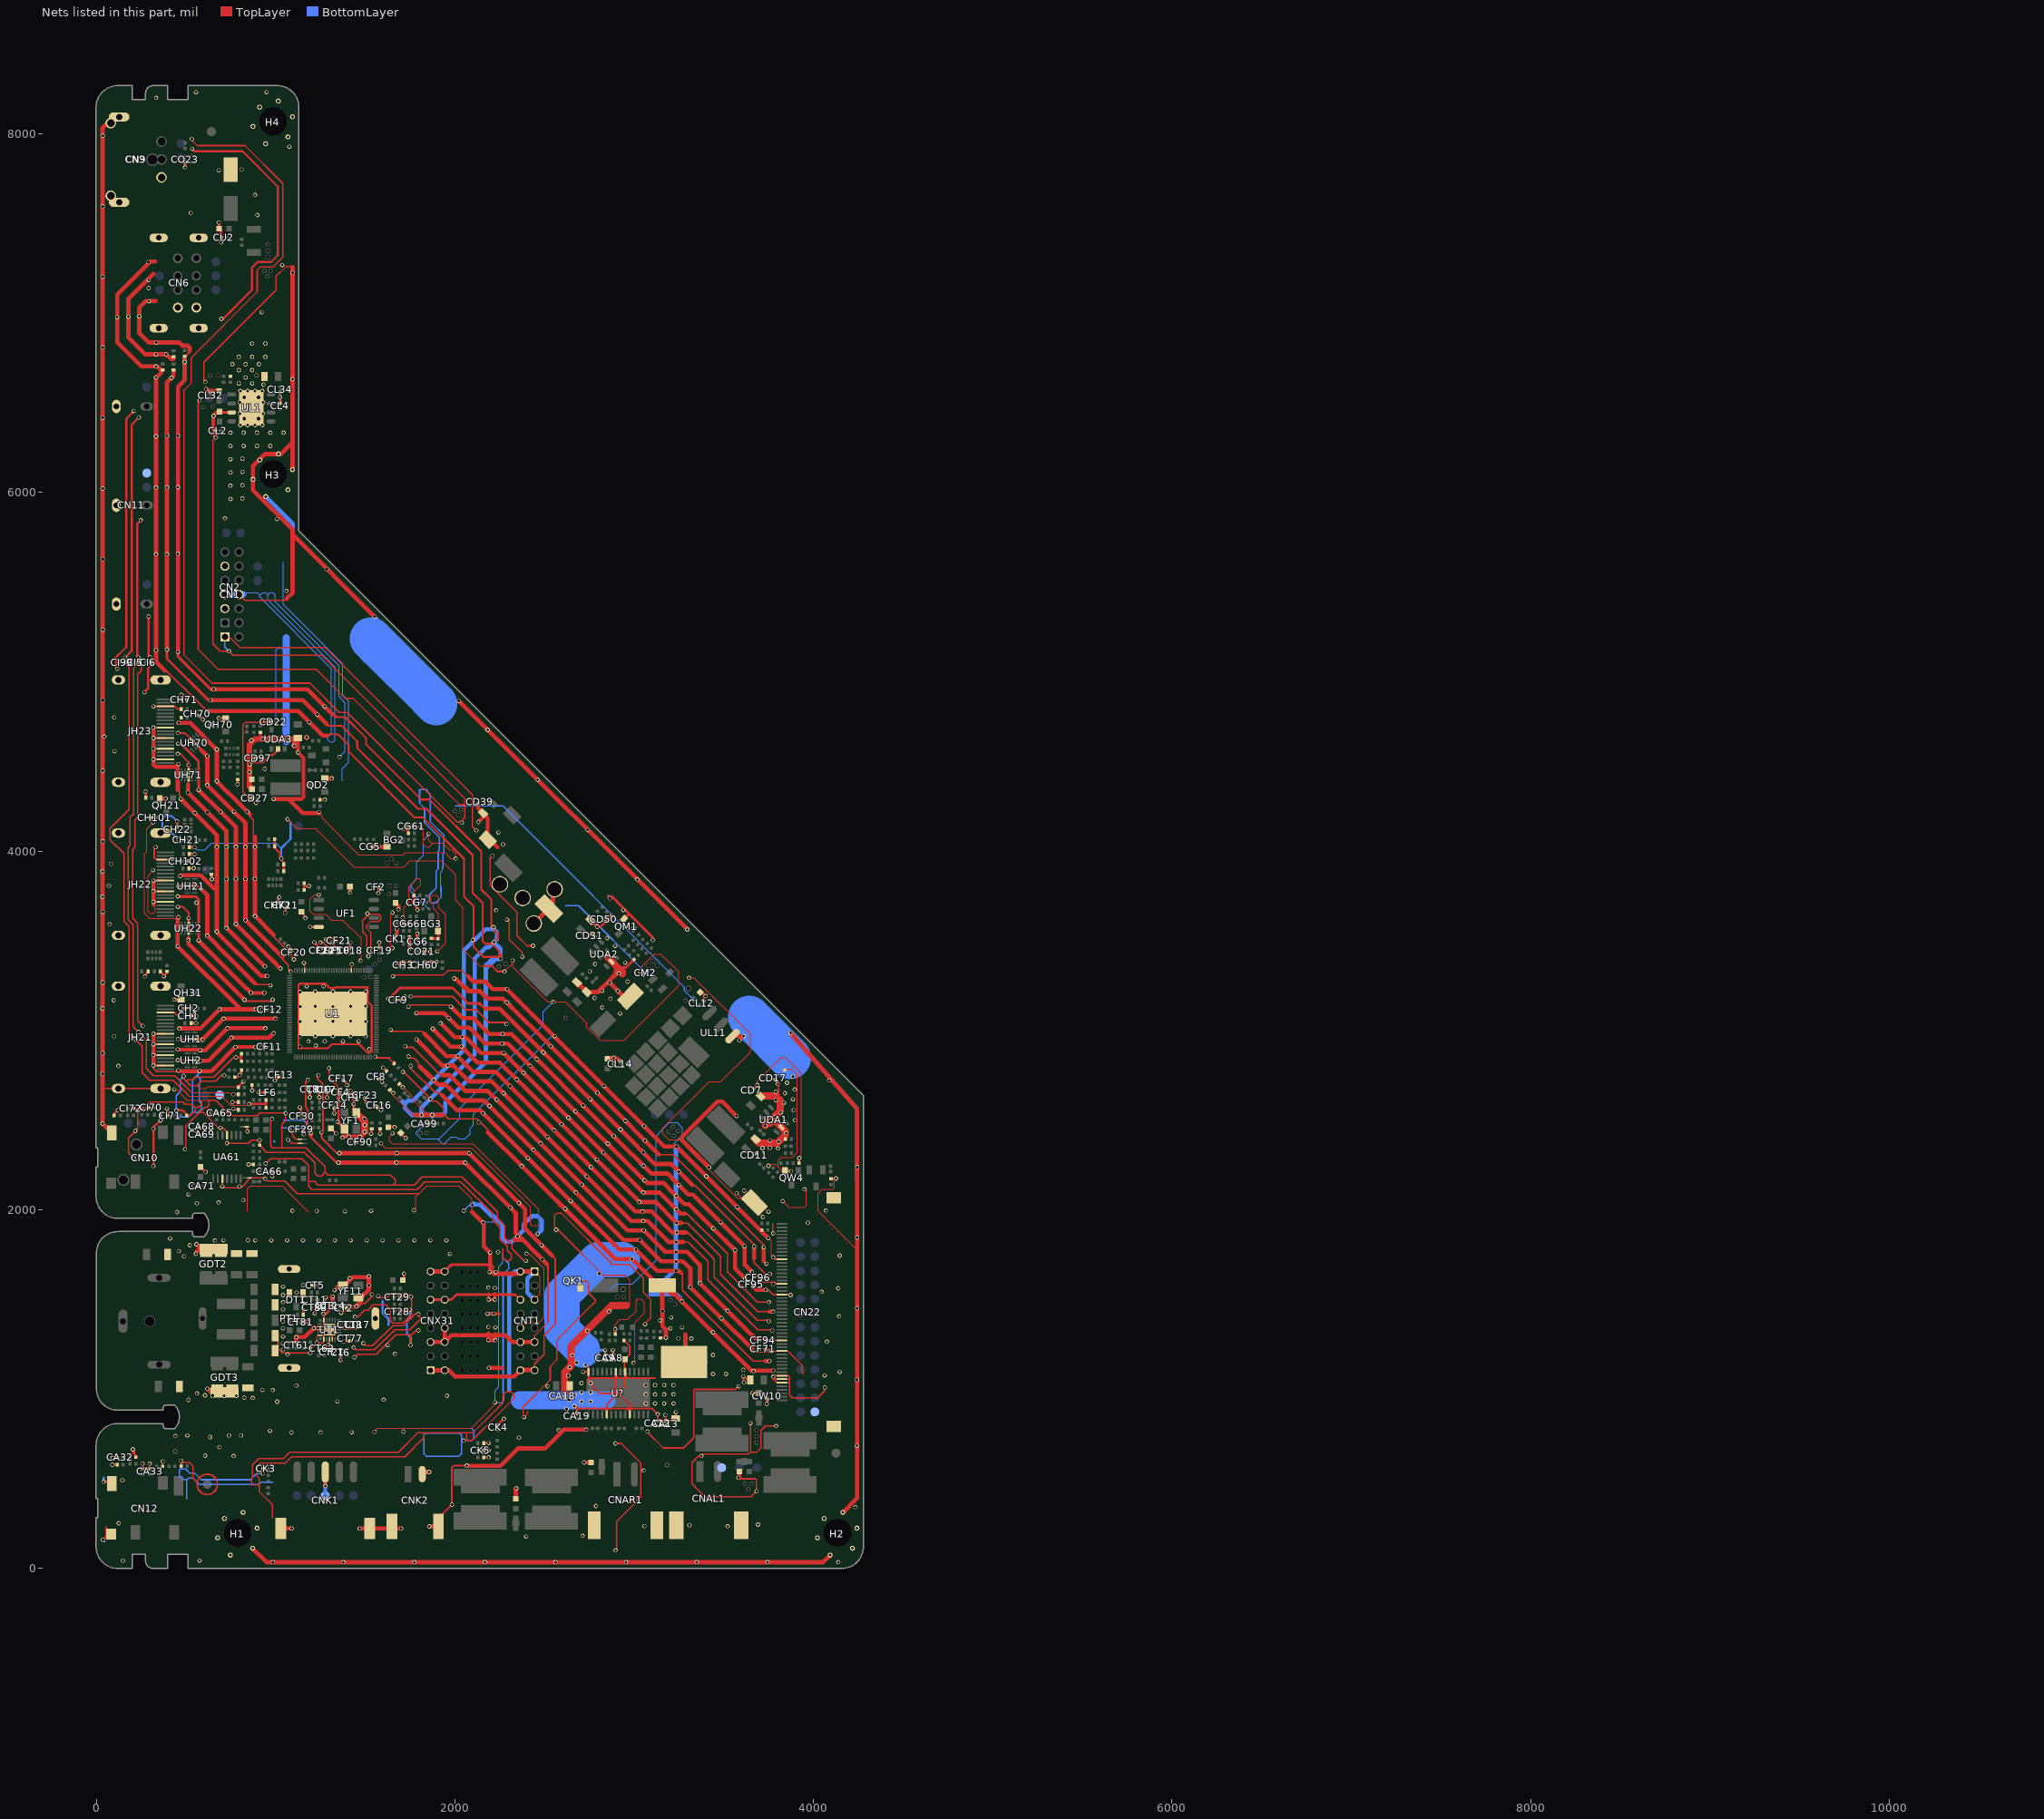
[diagram p0: the nets of this part, all layers, seen from the top]
# Altium PCB MISC105950.PcbDoc (part 9 of 15)
Units mil, origin at the board's own origin, x right, y up, seen from the top; angles counter-clockwise.
Board outline 4280.62 x 8272.76 mil, 2 copper layers (TopLayer, BottomLayer), stack 61.855 mil thick; 541 components, 268 nets, 2324 pads, 1157 vias.

## Via types
v1: diameter 23.62, hole 15.75, TopLayer to BottomLayer, tented both sides, 1087 vias
v2: diameter 23.62, hole 15.75, TopLayer to BottomLayer, 51 vias
v3: diameter 27.56, hole 19.68, TopLayer to BottomLayer, 15 vias
v4: diameter 31.5, hole 19.68, TopLayer to BottomLayer, tented both sides, 4 vias

## Nets (pads, with @x,y where several pads share a name; then routed paths per layer and width w, separated by ;. In a path a pad name is that pad's centre, name@x,y a point inside that pad or via, vN(x,y) a via of type N, cw(c..) or ccw(c..) an arc to the next point about the centre after c; other vN are vias at no path point) (continued)
GND: (continued)
  TopLayer w20: v1(453.5,2893) 455,2891.5 575.05,2891.5 v1(577.99,2888.56) ; v1(453.5,3747.33) 455,3745.83 528.17,3745.83 ; v1(622.51,4780.5) 654,4780.5 ; v1(652.81,6427.32) 651,6425.5 651,6354.27 ; CL2.1@658,6347.27 658,6314.5 v1(665.5,6307) ; CL2.1@660.27,6345 651,6354.27 ; 668,6447 651,6430 651,6354.27 ; v1@862.77,3207.5 935.12,3207.5 v1(936.93,3209.31) ; CD54.2@1123,4629.94 v1(1123,4549.75) 1154.65,4518.11 1154.65,4302.07 1142.95,4290.37 ; v1(1275.9,457.78) CNK1.3@1275.9,535.5 ; CG5.1@1542.23,4024 BG2.E@1620.5,4024 ; CF15.1@1668,3710.19 1684.5,3693.69 v1(1684.5,3674.5) ; CK1.1@1670.16,3527.73 1675,3532.57 v1(1675,3566) ; v1@1745.23,3452.73 RF13.2@1745.23,3518.5 ; CG6.1@1790,3513.73 v1(1790,3540.5) ; CD39.2@2126.67,4262.67 2126.67,4240.55 2182.29,4184.92 DM4.A@2182.29,4063.29 2193.71,4063.29 2237.5,4019.5 ; v1(2130,4162.5) 2156.11,4188.61 CD96.1@2156.11,4211.11 ; 2581.67,2029.67 2591.59,2019.75 2593.16,2019.75 2624.96,1987.96 ; v1(2615.04,2003.23) 2624.96,1993.32 2624.96,1987.96 ; v1(2719.69,588.81) CA22.1@2759,588.81 ; CD30.1@2754.89,3615.39 v1(2792.78,3577.5) ; 2760.41,1852.5 2727.96,1884.96 ; 2890.91,1722 2727.96,1884.96 ; UL11.1@3548.09,2967.53 v1(3609.97,2967.53) v1(3586,2943.5) v1(3586,2943.5) ; v1(3580.19,503.94) 3585.69,509.44 CA21.2@3585.69,537.5 ; v1@3659.31,975.31 CA20.1@3693.5,975.31 ; 2624.96,1987.96 2727.96,1884.96
  TopLayer w21: v1@775.81,2907 884,2907 v1(885.5,2905.5)
  TopLayer w23: v1(467.24,3861) 470.96,3864.71 580.52,3864.71 581.02,3865.21 ; v1@3755.87,1640.51 v1@3755.99,1640.63
  TopLayer w24: CN10.2@84.65,2427.17 v1(32.5,2479.31) 32.5,8033.88 94.51,8095.88 CN3.3@114.16,8095.88 ; 316.05,7218.88 177,7079.82 177,6865.45 271.07,6771.38 v1(388.82,6771.38) 413.55,6746.65 429.5,6746.65 ; v1@317.94,2803.15 317.94,2945.5 ; 317.94,2965.56 317.94,2945.5 ; v1@317.94,2979.56 317.94,2945.5 ; 317.94,3700.81 317.94,3741.5 ; v1@317.94,3716.54 317.94,3741.5 ; 317.94,3819.89 317.94,3799.83 ; v1@317.94,3833.89 317.94,3799.83 ; 317.94,4674.22 317.94,4654.16 ; v1@317.94,4688.22 317.94,4654.16 ; 326,7289.38 300.29,7289.38 114.66,7103.75 114.66,6839.22 249.5,6704.38 311.5,6704.38 ; v1@327.5,6704.38 311.5,6704.38 ; 331,7068.38 274.95,7068.38 238,7031.43 238,6890.71 291.84,6836.88 462,6836.88 479.91,6818.97 508.87,6818.97 518.83,6809.01 518.83,6791.03 ; 332,5054.13 380.56,5005.56 ; 332,5060.49 v1(332,6028) 332,6574 ; v1@332,6640.53 332,6574 ; QH21.E@351.5,4292.5 v1(385.5,4292.5) ; v1(393,5124) v1(393,6028) 393,6614.8 429.5,6651.3 429.5,6675.15 ; 452.48,4340.14 452.48,4390 ; 452.48,4353 452.48,4390 ; 452.48,4470.01 330.9,4470.01 317.94,4482.97 317.94,4654.16 ; v1(454,5110.28) v1(454,6029.5) 454,6589.53 491,6626.53 491,6749.65 ; v1@457.09,2771.87 591.5,2771.87 ; v1(457.1,3630.83) 452.48,3626.2 v1(452.48,3467.89) 802.87,3117.5 809.5,3117.5 ; v1(457.1,4485.16) 452.48,4480.54 452.48,4390 ; v1(457.49,4715.33) 521.94,4715.33 v1(670.48,4566.79) v1(670.48,4389.94) 814.46,4245.96 ; v1(460.88,3008.88) 462.88,3010.88 529.32,3010.88 579.88,3010.88 v1(686.5,3117.5) 809.5,3117.5 ; v1(470.11,4290.5) v1(547.8,4212.8) ; 510.05,4250.55 v1(547.8,4212.8) ; 510.1,4372.84 v1(510.1,4325.46) v1(619.03,4216.53) 724.5,4111.06 v1@724.5,4034 ; v1(512,3502.5) 512,3483.32 ; 512,3515.37 512,3483.32 ; 539.5,3865.21 581.02,3865.21 654.24,3792 670.66,3792 ; v2@556,1762 556.5,1762 574.17,1779.67 GDT2.2@653,1779.67 ; v2(556,1806) 557.01,1806 CT52.2@608.95,1754.06 ; v1(569.16,3501.11) 821.89,3248.39 ; v1(569.16,4341.36) v1(691.51,4219.01) 777.5,4133.02 v1(777.5,4023.5) v1(777.5,3844.5) v1(777.5,3592.58) 928.04,3442.04 ; v1(574.5,2771.87) 591.5,2771.87 ; v1@577.99,2829.5 623.36,2829.5 ; v1(577.99,2888.56) 607.46,2888.56 v1(730.41,3011.5) v1@932,3011.5 ; 577.99,2947.5 v1(591.45,2947.5) v1(708.45,3064.5) v1(998.39,3064.5) ; v1@580.22,3791.06 617.66,3753.63 v1(617.66,3527.57) 734,3411.23 ; v1(581.5,2829.5) 623.36,2829.5 ; 581.57,4566.07 v1(617.48,4530.15) v1(617.48,4367.98) v1(765.98,4219.48) 830.5,4154.97 v1(830.5,3844.5) v1(830.5,3614.54) 1036.74,3408.3 ; v1(610.5,6578) 621.43,6567.07 CL31.2@683.93,6567.07 ; v2(617.5,1000) 618.5,1000 639.17,979.33 GDT3.2@714.5,979.33 ; v1@623.5,4780.5 1125.88,4780.5 1262.38,4644 1285,4644 ; v1(636,4841.5) 1151.15,4841.5 1284.96,4707.69 ; v1@643.43,4902.5 675,4902.5 ; v1@661.88,4902.5 675,4902.5 ; v1@670.66,4017.5 670.66,4038 ; v1@724.5,4019.5 v1@724.5,4034 ; 766.01,3379.22 734,3411.23 ; v1(774.31,2905.5) 640.69,2771.87 591.5,2771.87 ; v1(824.82,3170.5) 512,3483.32 ; v1(841.21,4219.21) 814.46,4245.96 ; 846.77,3223.5 821.89,3248.39 ; 854.96,4205.46 814.46,4245.96 ; v1(860.77,3209.5) 821.89,3248.39 ; H1.5@870.29,110.12 947.91,32.5 4053.17,32.5 H2.6@4092.52,71.85 ; 882.91,3262.31 734,3411.23 ; 883.5,4079 v1(883.5,3636.49) 989,3531 ; v1(888,3117.5) 809.5,3117.5 ; v1@938.51,3011.5 v1@932,3011.5 ; v1(939.01,3356.12) v1(724.5,3570.63) v1@724.5,4034 ; v1(941.56,3011.5) v1@932,3011.5 ; v1(951.21,3303.12) 917.06,3303.12 v1(670.66,3549.52) 670.66,3792 ; 971.26,3398.82 928.04,3442.04 ; 971.5,2966.5 963.51,2958.5 ; v1(988.51,2983.5) 963.51,2958.5 ; v1@1025.5,3344.58 928.04,3442.04 ; CNK1.7@1027.87,220.54 v1(1088.54,220.54) ; 1060.5,5407.5 1093.48,5440.48 1093.48,5727.5 ; v1(1092.85,7225.5) 1092.85,7177 ; 1092.85,7258.5 1092.85,7177 ; 1093.48,5712.42 1093.48,5727.5 ; 1093.48,5764.6 v1(1550.19,5307.9) ; H3.4@1093.48,6130.55 1092.85,6131.19 1092.85,6280.38 ; 1115,1270 cw(c1117.41,1272.41) 1114,1272.41 v1(1114,1288) 1115.12,1289.12 1161.62,1289.12 1210.03,1337.53 v1(1212.89,1337.53) ; 1142.95,4290.37 v1(987.08,4290.37) 1070.65,4290.37 1149.53,4211.5 ; CT81.2@1159.5,1373.5 v1(1181,1373.5) ; 1194.5,2415.86 v1(1194.5,2429) ; 1206.06,4211.5 1149.53,4211.5 ; v1(1241.5,4217) 1241.5,4212.5 1240.5,4211.5 1149.53,4211.5 ; 1315.21,4763.71 v1(1272.21,4806.71) 1176.42,4902.5 675,4902.5 ; 1315.5,1499 1317,1500.5 v1(1317,1514.5) 1317,1489.5 1317.5,1489 ; v1@1315.5,1504.97 v1@1315.5,1515.1 ; 1340,1562 1354.96,1576.96 1383.69,1576.96 1429.23,1622.5 ; v1(1348.86,2261.5) v1(1672.5,2261.5) v1(2057.1,2261.5) v1(2309.05,2009.55) ; v1(1354,2314.5) 1407.5,2314.5 ; 1370.81,2314.5 1407.5,2314.5 ; v1(1371.66,2401.41) 1377.07,2406.83 v1(1407.5,2406.83) ; v1(1411.42,1616.43) 1423.16,1616.43 1429.23,1622.5 ; v1@1413,2406.5 1477.05,2406.5 1488.15,2417.6 1488.15,2425.97 v1@1490.09,2427.91 ; v1(1450.48,1460) 1470.31,1479.83 1470.31,1510.04 1476.63,1510.04 1519,1552.4 v1(1519,1577) 1519,1610 ; v1(1467.04,220.54) 1489.5,220.54 ; v1(1519,1626) 1519,1610 ; CNK1.6@1523.93,220.54 1489.5,220.54 ; v1(1699.04,220.54) 1489.5,220.54 ; 1777.52,2527.31 1846,2527.31 ; v1@1783.72,3096 1937.56,3096 1994.28,3039.28 ; v1(1784.88,2948.88) 1931.07,2802.68 ; 1805.31,2798.33 1805.31,2797.92 1847.61,2755.61 ; CNK2.2@1816.58,523.69 1828.39,535.5 v1(1855.5,535.5) ; 1828.35,2980.35 1953.03,2855.68 v1(2013.64,2855.68) 2102.13,2767.19 2227.47,2767.19 2328.83,2665.83 ; v1(1855.65,232.35) CNK2.4@1907.13,232.35 ; CNX31.1@1863.21,1102.99 1966.51,1102.99 ; CNX31.5@1863.21,1260.47 CNX31.6@1941.95,1260.47 ; CNX31.15@1863.21,1654.17 CNX31.16@1941.95,1654.17 ; v1(1873,2527.31) 1846,2527.31 ; v1(1875.5,3008.16) 1974.98,2908.68 v1(2035.6,2908.68) 2124.09,2820.19 2249.42,2820.19 2367.56,2702.06 ; v1(1880.5,2723) 1880.23,2723 1847.61,2755.61 ; v1(1919.24,3039.37) 1996.93,2961.68 ; 1924.32,2640.32 2011.13,2553.5 2139.46,2553.5 2187.48,2505.48 ; 1928.92,2749.68 1969.74,2749.68 2058.23,2661.19 2183.56,2661.19 2251.38,2593.38 ; 1931.5,2527.31 1846,2527.31 ; CNX31.2@1941.95,1102.99 1966.51,1102.99 ; CNX31.8@1941.95,1339.21 CNX31.6@1941.95,1260.47 ; 1955.3,3078.27 1994.28,3039.28 ; v1(1958,2802.68) 1931.07,2802.68 ; v1(1977.25,3131.27) 2040.84,3067.68 2056,3067.68 ; v1(1995,3289) 1999.5,3284.5 2006.99,3284.5 2073.49,3218 2081.05,3218 ; 2001.82,1067.68 1966.51,1102.99 ; v1(2020.83,4837.25) v1(3295.54,3562.54) ; v1(2040.5,2961.68) 1996.93,2961.68 ; 2041.32,3067.68 2056,3067.68 ; 2063.27,3235.77 2081.05,3218 ; v1(2065.5,571.5) 2066.71,570.29 2254.36,570.29 2350.89,666.82 2502.42,666.82 2607.35,771.75 v1(2732.25,771.75) ; 2077.5,3296.5 2103,3271 2169.93,3271 2211.24,3229.69 v1(2289.64,3229.69) 2540.69,2978.64 v1(2830.92,2688.42) 3167.83,2351.5 v1(3235.87,2351.5) v1(3401.44,2185.94) v1(3574.69,2012.69) v1(3746.74,1840.63) ; 2094.93,1986.79 2160.66,1921.07 2160.66,1795.34 v1(2196,1760) 2196,1664.5 2219,1641.5 2351.86,1641.5 CNT1.2@2364.47,1654.11 CNT1.1@2433.5,1654.11 ; v1(2156.98,2535.98) 2187.48,2505.48 ; 2168.66,3120.68 2248.75,3120.68 2320.71,3048.71 2518.71,2850.71 ; 2183.46,2430.71 v1(2371.83,2242.33) 2592.42,2021.75 ; 2184.5,1299 2234.5,1299 ; 2185.5,1308 v1(2185.5,1271.5) 2219.5,1271.5 2223.5,1275.5 2223.5,1305.5 ; v1(2189.5,1116.5) 2261,1116.5 ; v1(2191.85,2577.95) 2212.4,2557.4 ; v1(2192.5,1651) v1(2226.5,1651) ; 2194,1688 2196,1690 ; v1(2231.38,2613.38) 2251.38,2593.38 ; v1(2253.66,3399.16) 2253.66,3416.16 ; v1(2263.5,2926.19) 2293.33,2926.19 ; v1(2265,2979.19) 2293.5,2979.19 ; v1(2270.85,2648.85) 2294.85,2624.85 ; 2284.5,1296 2320.09,1260.41 ; v1(2306.83,2687.83) 2328.83,2665.83 ; 2317.63,2000.96 v1(2309.05,2009.55) ; 2323.5,1995.1 v1(2309.05,2009.55) ; CA23.2@2339.05,386.81 2339.05,441.55 v1(2342,444.5) ; v1(2344.81,2724.81) 2367.56,2702.06 ; v1(2348.76,1850.22) 2331,1832.46 2331,1831.5 2377,1831.5 ; v1(2356.77,2036.77) 2368.52,2025.02 ; v1(2382.28,2762.28) 2410.03,2734.53 ; v1(2418.01,2801.51) 2433.01,2786.51 ; CNT1.15@2441.64,1104.5 2366.04,1104.5 2330.04,1068.5 2001,1068.5 1966.51,1102.99 ; CNT1.11@2443.21,1260.41 2320.09,1260.41 ; v1(2456.24,2838.24) 2472.99,2821.49 ; 2473,1735.5 2444,1764.5 ; v1(2483.33,1800.14) 2460.48,1822.98 ; v1(2493.21,2876.21) 2518.71,2850.71 ; 2512,1696.51 2444,1764.5 ; 2541.48,1741.98 2460.48,1822.98 ; 2569.25,2048.75 2894.01,1724 2951.5,1724 ; 2891.74,1724 2951.5,1724 ; 2934.35,2210.22 2925.03,2219.53 ; v1(3046,1989) 3005.66,1989 ; v1(3049.5,1936) 2983.71,1936 ; v1(3056.68,2162.84) 2996.51,2223.01 ; v1(3059.94,2384.44) 3041.94,2402.44 ; 3137.38,2307 3041.94,2402.44 ; v1@3156.5,1431 EA33.2@3156.5,1577.5 ; v1@3156.5,1441.5 EA33.2@3156.5,1577.5 ; v1(3157,1433) 3157,1348.97 3176.23,1329.74 v1(3176.23,1284.27) ; v1@3231.7,2078.7 3216.2,2094.2 ; v1(3233,1657.87) 3196.5,1657.87 ; v1(3233,1710.87) 3187,1710.87 ; v1(3233,1763.87) 3203,1763.87 ; v1(3233,1818.55) 3192.04,1818.55 ; v1(3233.52,2001.92) 3211.47,2023.97 ; v1(3236.5,1871.55) 3213.99,1871.55 ; v1(3248.4,2211.91) 3238.56,2221.75 ; v1(3248.66,2136.69) 3233.68,2151.68 ; 3259.45,1647.69 3249.27,1657.87 3196.5,1657.87 ; 3262,1924.55 v1(3235.94,1924.55) 3118.49,2042 v1(3027.61,2042) v1(2791.06,2278.56) v1(2594.31,2475.31) 2367.56,2702.06 ; 3263.96,2388.46 3276.46,2375.96 v1(3417.46,2234.96) 3403.71,2248.71 ; v1(3265.86,1487.86) 3251.86,1501.86 ; 3266.45,2391.02 3266.45,2404.61 3463.21,2601.37 3490.13,2601.37 v1(3570,2521.5) ; 3272.5,1818.55 3192.04,1818.55 ; 3283.15,1977.55 3257.9,1977.55 3211.47,2023.97 ; HSA1.1@3285,1148 3285,1302.5 ; 3287.32,1871.55 3213.99,1871.55 ; 3312.45,1626.5 3312.45,1669.64 ; 3323.76,2136.55 3238.56,2221.75 ; 3615.45,1692.64 v1(3656.28,1651.81) ; 3615.45,1693.5 v1(3615.45,1795.14) v1(3481.05,1929.55) 3327.05,2083.55 3301.8,2083.55 3233.68,2151.68 ; v1(3618.53,1614.61) 3562.45,1670.69 v1(3562.45,1773.19) v1(3441.07,1894.57) 3305.1,2030.55 3279.85,2030.55 3216.2,2094.2 ; 3660.25,1219.34 v1(3486.04,1393.54) v1(3312.45,1567.13) 3312.45,1669.64 ; 3668.45,1725.88 3668.45,1773.5 ; v1@3668.45,1791.5 3668.45,1773.5 ; v1(3668.45,1793.06) 3668.45,1773.5 ; 3669.63,1563.52 3681.63,1551.51 v1(3733.68,1551.51) ; 3673.91,1280.63 v1(3519.52,1435.02) v1(3365.45,1589.09) 3365.45,1691.59 3293.18,1763.87 3203,1763.87 ; 3722,1711.96 3722,1778 v1(3722,1790.42) ; 3730,1154.44 v1(3753.55,1154.44) ; 3753.55,1430.03 3774.85,1430.03 v1(3775,1429.88) ; v1(3775,1101.38) v1(3775,1101.38) 3753.5,1101.44 ; v1(3775,1733.38) v1@3775.92,1734.3 ; v1@3775.5,1101.44 3753.5,1101.44 ; v1(3871.77,2984.83) 4243.09,2561.99 4243.09,1784 4243.09,969.38 ; H2.3@4163.39,310.04 4242.46,389.11 4242.46,968.74 4243.09,969.38 ; 4243.09,945.88 4243.09,969.38 ; 311.5,6704.38 338.51,6704.38 360.42,6682.46 360.42,6668.49 332,6640.07 332,6574 ; 317.94,3741.5 317.94,3775.59 317.94,3799.83 ; v1(547.8,4212.8) 670.66,4089.95 670.66,4038 ; 623.36,2829.5 v1(752.36,2958.5) 963.51,2958.5 ; 670.66,3792 670.66,4038 ; 1092.85,6280.38 1027.04,6214.57 937.78,6214.57 872.05,6148.84 872.05,6014.33 1093.48,5792.89 1093.48,5727.5 ; 1092.85,6280.38 1092.85,7177 ; 1407.5,2314.5 v1(1674,2314.5) v1(2079.05,2314.5) 2368.52,2025.02 ; 1429.23,1622.5 1506.5,1622.5 1519,1610 ; 1847.61,2755.61 1906.55,2696.68 1947.78,2696.68 1975.23,2669.23 2036.27,2608.19 2161.61,2608.19 2212.4,2557.4 ; 1931.07,2802.68 1991.69,2802.68 2080.18,2714.19 2205.52,2714.19 2294.85,2624.85 ; CNX31.6@1941.95,1260.47 1980.48,1299 2234.5,1299 ; 1994.28,3039.28 2018.89,3014.68 2079.5,3014.68 2103.59,2990.59 2167.99,2926.19 2293.33,2926.19 ; 1996.93,2961.68 2057.55,2961.68 2071.36,2947.86 2146.04,2873.19 v1(2271.38,2873.19) 2410.03,2734.53 ; 2056,3067.68 2101.46,3067.68 2189.95,2979.19 2293.5,2979.19 ; 2081.05,3218 2139.51,3218 2180.82,3176.69 2267.69,3176.69 v1(2289.44,3154.94) v1(2533.44,2910.94) v1(2794.44,2649.94) v1(2949.94,2494.44) 3041.94,2402.44 ; 2187.48,2505.48 v1(2406.98,2285.98) v1(2644.48,2048.48) 2915.96,1777 v1(3008.73,1777) 3127.86,1657.87 3196.5,1657.87 ; 2212.4,2557.4 v1(2436.65,2333.15) v1(2674.4,2095.4) 2939.8,1830 v1(3030.68,1830) 3149.81,1710.87 3187,1710.87 ; 2234.5,1299 2281.5,1299 2320.09,1260.41 ; 2251.38,2593.38 v1(2476.38,2368.38) v1(2706.13,2138.63) 2961.75,1883 v1(3052.63,1883) 3171.76,1763.87 3203,1763.87 ; 2293.33,2926.19 2433.01,2786.51 ; 2293.5,2979.19 2315.28,2979.19 2472.99,2821.49 ; 2294.85,2624.85 v1(2514.6,2405.1) v1(2735.35,2184.35) 2983.71,1936 ; v1(2309.05,2009.55) 2338,1980.6 2338,1870.51 2377,1831.5 ; 2328.83,2665.83 v1(2552.58,2442.08) v1(2758.08,2236.58) 2890.44,2104.22 3005.66,1989 ; 2368.52,2025.02 2391,2002.55 2391,1892.46 2460.48,1822.98 ; 2377,1831.5 2444,1764.5 ; 2410.03,2734.53 v1(2632.53,2512.03) v1(2826.03,2318.53) 2925.03,2219.53 ; 2433.01,2786.51 v1(2672.01,2547.51) v1(2852.01,2367.51) 2996.51,2223.01 ; 2472.99,2821.49 v1(2714.49,2579.99) v1(2884.99,2409.49) 3093.47,2201 3184.35,2201 3233.68,2151.68 ; 2518.71,2850.71 v1(2754.46,2614.96) v1(2923.46,2445.96) 3115.43,2254 3206.3,2254 3238.56,2221.75 ; 2925.03,2219.53 v1(3049.57,2095) 3140.44,2095 3211.47,2023.97 ; 2951.5,1724 v1(2986.77,1724) 3133.27,1577.5 EA33.2@3156.5,1577.5 ; 2983.71,1936 3074.58,1936 3192.04,1818.55 ; 2996.51,2223.01 3071.52,2148 3162.4,2148 3216.2,2094.2 ; 3005.66,1989 3096.54,1989 3213.99,1871.55 ; EA33.2@3156.5,1577.5 3203.73,1530.27 3223.45,1530.27 3251.86,1501.86 ; 3187,1710.87 3271.22,1710.87 3312.45,1669.64 ; 3251.86,1501.86 v1(3438.86,1314.86) 3652.29,1101.44 3753.5,1101.44
  TopLayer w25: QD2.E@1273,4406 v1(1312,4406) ; pad.VIA5@2439.5,3595.5 2439.5,3596.61 EA34.2@2518.44,3675.56 ; EA34.2@2546.5,3702.5 pad.VIA5@2546.5,3782 ; CD53.2@2679.99,3267.29 CD57.2@2733.99,3213.29 2796.79,3213.29 v1@2855.5,3272 ; 2892.89,3309.39 2898,3314.5 ; 2898,3349.99 2898,3314.5 ; EA1.2@2953.44,3174.06 v1@2855.5,3272 ; v1@2855.5,3272 2898,3314.5
  TopLayer w30: v1@853.65,4493.49 853.65,4512.5 ; 853.65,4533.9 853.65,4512.5 ; CD26.1@866.94,4345.41 853.65,4358.69 v1(853.65,4441) 853.65,4512.5 ; v1(1103,4588) 1103,4606 ; CD54.2@1103,4626 v1(927,4626) 885,4626 853.65,4594.65 853.65,4512.5 ; v1@1171,4634 v1(1172,4634)
  TopLayer w40: YF1.2@1449.5,2538.81 1496.15,2492.16 v1(1496.15,2433.97) ; 2610.86,996 2610.86,1091.5 2646.86,1127.5 2646.86,1237.82 2874.04,1465 2956,1465 ; 2848.62,3410 2932.5,3326.12 2932.5,3313.5 ; CD99.2@3675.5,2391.06 3697.06,2369.5 3796.5,2369.5 3841.73,2414.73 3841.73,2437.27 3785.54,2493.46 3777.5,2493.46 ; CD77.1@3705.61,2634.31 3787.69,2634.31 3813.5,2608.5 3813.5,2550.5 v1(3731,2468) ; v1@3756.46,2493.46 3757.54,2493.46 3757.54,2482.14
  TopLayer w50: HSA1.1@3285,1148 HSA1.1@3383,1148
  BottomLayer w5: v1@536.02,3904.02 v1(541.9,3904.02) ; v1@542.73,3942.5 v1@543.73,3943.5 ; v1(545.46,4021.74) 559.7,4007.5 603.58,4007.5 640.58,4044.5 734,4044.5 ; 745,4044.5 734,4044.5 ; 1029.85,4015.11 1000.45,4044.5 734,4044.5 ; v1(1550,759.5) 1570.35,779.85 2090.96,779.85 ; v1@1647,3660.17 v1(1651.16,3656.01) ; v1@1677.5,3371.5 v1@1678,3371 ; v1(1712,4122.5) v1@1712,4125.5 ; 1744.5,3467 1745,3466.5 ; 1756.5,3803.5 1750.61,3797.61 1750.61,3778.89 1845.75,3683.75 ; 1770,3782.5 1756.5,3796 1756.5,3814.31 1786,3843.81 1786,3921.5 ; 1786,3913.38 1786,3921.5 ; v1@1789.5,3541 v1(1790,3540.5) ; v1@1852,4089 1823.19,4060.19 1823.19,3976.33 1786,3939.14 1786,3921.5 ; v1(1873,2478.5) 1832.18,2478.5 1783.36,2429.68 1783.36,2423.32 1811.49,2395.19 1894.5,2395.19 ; 1919.81,3774.31 1919.81,3880.9 1930.5,3891.59 1930.5,3914 1932,3915.5 ; v1(2157.5,1928.5) 2160.12,1931.12 2233.44,1931.12 2235.28,1929.28 ; 2265.5,1732.57 2265.5,1703.62 2243,1681.12 2243,1010.89 2222.61,990.5 v1(2222.61,924.66) 2261.66,924.66 2270.69,933.69 ; v1(2548,3158) 2492.69,3102.69 2492.69,3030.54 2025.17,2563.02 2025.17,2507.49 1912.86,2395.19 1894.5,2395.19 ; v1(2555.5,2967) 2539.45,2967 2103.17,2530.71 2103.17,2471.39 2083.5,2451.72 2083.5,2422 2055.5,2394 2018.81,2394 2008,2404.81 1977.12,2404.81 1942.5,2370.19 1926.5,2370.19 1901.5,2395.19 1894.5,2395.19
  BottomLayer w6: CN2.6@794.34,5431.32 803.33,5440.31 897.71,5440.31 909.31,5428.71 ; 1041.61,5614.23 1041.61,5374.59 1372.78,5043.42 1372.78,4869.96 1407,4835.74 1407,4496 1371.5,4460.5 1371.5,4390.5 ; 1329.81,4619.79 1318.21,4608.19 1301.79,4608.19 1290.19,4619.79 1290.19,4636.21 1309.78,4655.79 1309.78,5017.19 909.31,5417.66 909.31,5428.71 ; 1330,4618 1330.78,4618.78 1330.78,5025.89 954.81,5401.86 954.81,5428.71 ; v1(1355.5,4525) 1386,4555.5 1386,4827.04 1351.78,4861.26 1351.78,5034.72 994.81,5391.69 994.81,5428.71 983.21,5440.31 966.79,5440.31 955.19,5428.71 954.81,5428.71 ; v1(2460,1863.5) v1@2460,1867.5 ; 2870,1554.12 2899.88,1584 2989.51,1584 3121,1715.49 3121,2410.62 3194.88,2484.5 3237.12,2484.5 3268.45,2453.18 3268.45,2413.82 3223,2368.38 3223,2293.5 ; v1(3054.46,2465.14) 3065.59,2454.01 ; v1@3745,2241 v1(3748,2244) ; v1(4125.15,2172.73) v1@4125.15,2172.85 ; 909.31,5428.71 915.19,5428.71 926.79,5440.31 943.21,5440.31 954.81,5428.71 ; 1001.19,4742.29 1001.19,5121.71 1012.79,5133.31 1029.21,5133.31 1040.81,5121.71 1040.81,4742.29 1029.21,4730.69 1012.79,4730.69 1001.19,4742.29
  BottomLayer w7: v2@446.65,1985.65 v2(448.81,1985.65) ; v1(454.99,2776.5) 569.87,2776.5 v1(574.5,2771.87) 574.5,2762.72 560.14,2748.36 ; 491,2779 486,2774 v1(486,2743.5) 467,2724.5 467,2657.5 445.5,2636 v1(445.5,2553) 445.5,2523 452,2516.5 509,2516.5 535,2542.5 ; v1@763,2641.48 v1(763,2642.5) ; v1(978.5,2505) v1@978.5,2509 ; v1(1025.69,3344.37) v1@1033.63,3344.37 ; 1028.31,2455.19 1158.91,2455.19 1170.81,2467.09 1170.81,2483.91 1155.41,2499.31 1041.09,2499.31 ; v1(1092.5,2450) v1@1095.5,2450 ; v1@1093.23,3393.3 v1@1102.38,3393.3 ; 1121.8,2538.73 1126.46,2538.73 ; v1@1356,1423 v1(1364.5,1423) ; v1@1383,1337 v1(1384.5,1338.5) ; v1@1440.5,1403.5 v1(1442,1402) ; v1(1751.25,1243.02) v1@1751.25,1250.25 ; v1@2127.16,2491.12 v1(2132.48,2485.8) ; v1(2395,1714.5) v1@2395.5,1715 ; v1(3760,1268.88) v1@3760,1269.37 ; v1(3775,1584.88) v1@3775,1592.01 ; v1(3775.11,1067.56) v1@3777,1069.45 ; v1@3869,1523 v1(3872,1523) ; 535,2542.5 565.5,2542.5 585.19,2562.19 585.19,2591.53 572.69,2604.03 572.69,2703.41 579.31,2710.03 579.31,2729.19 560.14,2748.36 ; 535,2542.5 535,2723.22 560.14,2748.36
  BottomLayer w8: v2@76.5,615 114,615 v2(88,615) ; v2(297,582) v2@297.5,582 ; v2@368.5,594.5 v2(369,595) ; v2@471.5,595 v2(471.5,597.5) ; v1@478,2743.5 v1(486,2743.5) ; 502.5,384 502.5,489.5 515.5,502.5 538,502.5 574,466.5 877.57,466.5 906.5,466.5 918,478 982,478 ; 506.31,493.31 481.19,493.31 462.5,512 462.5,546.5 467.5,551.5 497.5,551.5 520.5,528.5 548.77,528.5 584.77,492.5 858,492.5 892,526.5 v2(928.5,526.5) ; v1@570.67,6514 v1(574,6514) ; v1@575,6514 v1@575.5,6514.5 ; CN1.1@715.6,5195.1 715.6,5137.93 v1(739.14,5114.39) ; v1@1155,3377 v1(1157,3377) ; v1@1158.16,3366.56 v1@1159.34,3367.74 ; v2(1294.25,1244.78) v2@1296.22,1244.78 ; v1@1423,3365.5 1423.5,3366 v1(1423.5,3368.5) ; v1@1467.64,3388.38 v1(1472.12,3388.38) ; v1@1534.5,3445.5 v1(1539,3445.5) ; v1@1649.94,3304.5 v1(1653.25,3301.19) ; 1844,4342.5 1836,4342.5 ; 1921.31,3802.5 1921.31,3739.88 1891.43,3710 1868.5,3710 1857.06,3721.44 1857.06,3755.83 1895.31,3794.09 1895.31,3891.05 1906,3901.74 1906,3998.76 1912.31,4005.07 1912.31,4076.19 1830,4158.5 1830,4238.5 1802,4266.5 1802,4342.5 1836,4342.5 ; 1932,3906.62 1932,3985 1938.31,3991.31 1938.31,4087.07 ; 1938.31,4041 1938.31,4087.07 ; 1999.66,4252.81 2265.97,4252.81 3278,3240.77 3278,3223.5 3323.24,3178.26 3332.76,3178.26 ; 2017.85,4162 v1@2030.5,4162 ; v1@2048.58,717.97 v1(2048.58,711.19) 2092.62,711.19 2104.81,723.38 2104.81,766 2090.96,779.85 ; v1(2048.98,1992.98) 2081,2025 v1(2094.93,2025) ; 2192,3958.5 2193,3957.5 ; 2257.5,1891 2264,1884.5 ; 2265.5,1763.5 2265.5,1732.57 2299,1699.07 2299,1669.08 2267.5,1637.58 2267.5,978.12 2270.69,974.93 2270.69,933.69 ; 2615.02,3695.11 2688.89,3695.11 3077,3307 ; v1@3775.11,1860.75 v1(3775.11,1867.15) ; 1836,4342.5 1860.5,4318 1860.5,4164.88 1938.31,4087.07 ; 1825.14,638.07 1839.49,623.71 2021.2,623.71 2035.55,638.07 2035.55,741.53 2025,752.09 1836,752.09 1825.14,741.22 1825.14,638.07
  BottomLayer w10: v1(317,2803) v1@317.94,2803.94 ; v1(317,2862) v1@317.94,2862.94 ; v1(317,2921.5) v1@317.94,2920.56 ; v1(317,2980.5) v1@318,2980.5 ; v1(317,4807) v1@321,4807 ; JH22.20@356.91,4100.4 366.96,4110.45 366.96,4182.46 379.74,4195.24 419.76,4195.24 v1(449.5,4165.5) ; v1@469.09,3121.09 v1(469.09,3123.27) ; v1@544,3943 v1@544,3943.5 ; v1@640,3840 v1(643,3843) ; v1(982.47,3170.31) v1@987.88,3164.9 ; v1@1174.78,2726.22 v1(1178,2723) ; v1@1188,2435.5 v1(1194.5,2429) ; v1@1234.04,2752.12 v1(1237.22,2748.94) ; v1@1237.09,2626.09 v1(1242.62,2626.09) ; v1@1554.5,2850.28 v1(1554.5,2852.5) ; v1@1597.86,2791.69 v1(1598.61,2791.69) ; v1@1745,3189 v1(1753,3189) ; v1@2633.5,935 v1(2636,937.5) ; v1(2727.87,1132.13) 2742.63,1132.13 ; v1@3072,756.16 v1@3072,765 ; v1(3231,869) v1@3232,868 ; v1(3659,975) v1@3662,978
  BottomLayer w11: v1@2092.5,3497.5 v1(2099,3504)
  BottomLayer w12: v1(35,157.5) 44,148.5 ; v1(39,480.5) 39,504.5 ; v2(87.5,576.5) v2@88.5,575.5 ; v1@160,5078.5 v1(160,5080) ; v1(269.5,3300) v1@269.5,3301.5 ; v1(272,4332) v1@274.65,4334.65 ; JH22.20@356.91,4100.4 419.91,4100.4 v1(456.94,4063.36) v1@458.64,4063.36 ; v1@433.5,3168.45 v1(433.5,3171) ; v1@545.46,4019.54 v1(545.46,4021.74) ; v1@554.5,3077.22 v1(555.91,3078.62) ; v1(785.84,4372.36) v1@789.29,4372.36 ; 853.65,4514.15 857,4517.5 ; v1@909,2386.5 v1(909,2387) ; v1(919.5,2905.5) v1@920.5,2905.5 ; v1(922,3117.5) v1@923,3117.5 ; v1(943,2256.5) v1@944,2257.5 ; v1@979,2185.5 v1(980,2185.5) ; 991,2380 991.5,2379.5 ; v1@1018,3740.5 v1(1019.29,3741.79) ; v1(1029.85,3958.74) 1029.85,4015.11 1081.98,4067.24 1081.98,4113.5 ; v1(1051.69,3655) v1@1052.19,3654.5 ; v1(1065,4177.5) 1081.98,4160.52 1081.98,4113.5 ; 1081.98,4143.26 1081.98,4113.5 ; v1(1156,2419) v1@1163.5,2426.5 ; v1(1164.5,3626.5) v1@1167.38,3629.38 ; v1(1192,3576.5) v1@1193,3577.5 ; v1(1248.5,3490) v1@1249,3490.5 ; v1@1285,2624.5 v1(1285.5,2624.5) ; v1(1335.87,2424.69) v1@1335.87,2427.94 ; v1(1468.68,2406.5) v1(1496.15,2433.97) ; v1(1494.57,2505.32) 1496.15,2503.74 v1(1496.15,2471.5) ; v1@1502.28,2594.1 v1(1510.5,2594.1) ; v1(1531.45,2422.6) v1@1534.35,2425.5 ; v1@1579.6,2422.6 v1(1582.14,2422.6) ; v1@1587.01,2553.01 v1(1587.01,2553.4) ; v1@1591.1,2711.6 v1(1592.97,2711.6) ; 1595.19,1488.81 1595.19,1423.05 1628,1390.24 1628,1357.5 ; v1(1720.18,1525.35) v1@1720.5,1525.03 ; v1(1724.35,2398.31) v1@1725.5,2397.17 ; v1(1747,1441) 1747,1392.02 1731.5,1376.52 1731.5,1306.76 1751.81,1286.45 v1@1751.81,1243.58 ; v1(1873,2478.5) v1@1873,2523.81 ; 2631.1,1215.9 v1@2840.5,1215.9